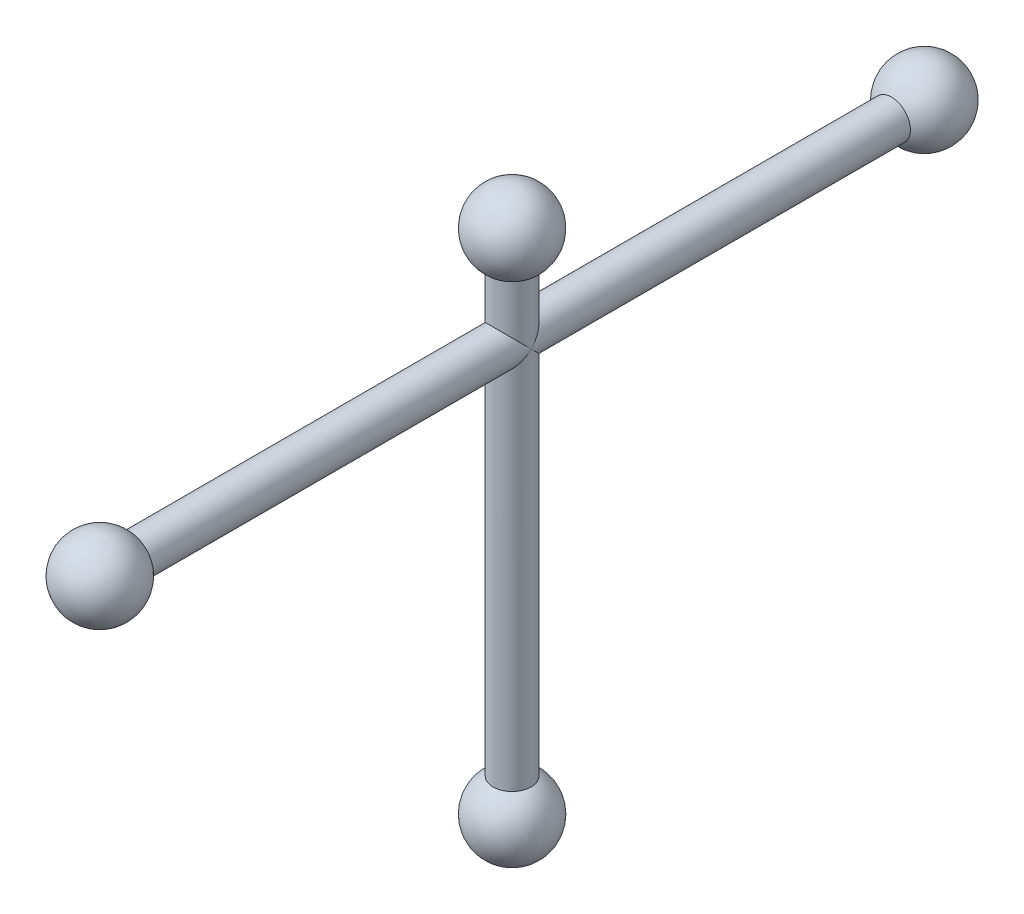
from build123d import *

# Parameters (mm, degrees)
SKETCH1_R           = 15
BOSS_EXTRUDE1_DEPTH = 300
SKETCH3_R           = 15
BOSS_EXTRUDE2_DEPTH = 50
BOSS_EXTRUDE3_START = -300
SKETCH5_R           = 15
BOSS_EXTRUDE3_DEPTH = 300


with BuildPart() as part:
    # Sketch1 → Boss-Extrude1 (new, symmetric)
    with BuildSketch(Plane.XY):
        Circle(SKETCH1_R)
    extrude(amount=BOSS_EXTRUDE1_DEPTH, both=True)

    # Sketch2 → Revolve1 (revolve)
    with BuildSketch(Plane(origin=(0, 0, 0), x_dir=(1, 0, 0), z_dir=(0, 1, 0))):
        with BuildLine():
            Line((0, 355), (0, 295))
            ThreePointArc((0, 295), (30, 325), (0, 355))
        make_face()
    revolve1 = revolve(axis=Axis((0, 0, -355), (0, 0, 1)))

    # Mirror1: Revolve1 across plane
    add(revolve1.mirror(Plane.XY))

    # Sketch3 → Boss-Extrude2 (add)
    with BuildSketch(Plane(origin=(0, 0, 0), x_dir=(1, 0, 0), z_dir=(0, 1, 0))):
        Circle(SKETCH3_R)
    extrude(amount=BOSS_EXTRUDE2_DEPTH)

    # Sketch4 → Revolve2 (revolve)
    with BuildSketch(Plane.XY):
        with BuildLine():
            Line((0, 105), (0, 45))
            ThreePointArc((0, 45), (30, 75), (0, 105))
        make_face()
    revolve(axis=Axis((0, 105, 0), (0, -1, 0)))

    # Sketch5 → Boss-Extrude3 (add)
    with BuildSketch(Plane(origin=(0, 0, 0), x_dir=(1, 0, 0), z_dir=(0, 1, 0)).offset(BOSS_EXTRUDE3_START)):
        Circle(SKETCH5_R)
    extrude(amount=BOSS_EXTRUDE3_DEPTH)

    # Sketch6 → Revolve3 (revolve)
    with BuildSketch(Plane(origin=(0, 0, 0), x_dir=(0, 0, -1), z_dir=(1, 0, 0))):
        with BuildLine():
            Line((0, -295), (0, -355))
            ThreePointArc((0, -355), (-30, -325), (0, -295))
        make_face()
    revolve(axis=Axis((0, -295, 0), (0, -1, 0)))


solid = part.part
